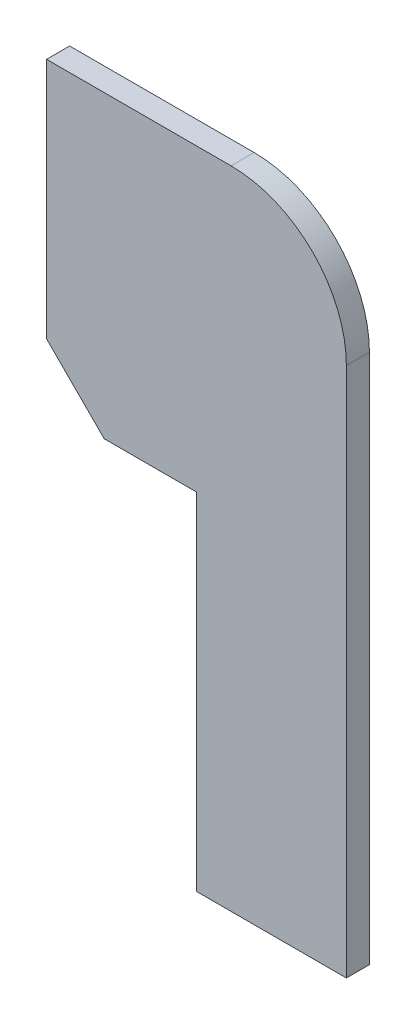
SolidWorks part; units mm, degrees
material "普通碳钢"
ref_plane "Front Plane" through (0, 0, 0) normal (0, 0, 1) x (1, 0, 0)
ref_plane "Top Plane" through (0, 0, 0) normal (0, 1, 0) x (1, 0, 0)
ref_plane "Right Plane" through (0, 0, 0) normal (1, 0, 0) x (0, 0, -1)
sketch "Sketch1" plane through (0, 0, 0) normal (0, 0, 1) x (1, 0, 0)
  line L0 (0, 175) -> (0, 280)
  line L1 (0, 280) -> (80, 280)
  line L2 (130, 230) -> (130, 0)
  line L3 (130, 0) -> (65, 0)
  line L4 (65, 0) -> (65, 150)
  line L5 (65, 150) -> (25, 150)
  line L6 (25, 150) -> (0, 175)
  arc A0 (80, 280) -> (130, 230) centre (80, 230) cw
  point P0 (0, 150)
  dimension "D5" = 50
  dimension "D1" = 280
  dimension "D2" = 150
  dimension "D3" = 65
  dimension "D4" = 130
extrude "Boss-Extrude1" add sketch "Sketch1" along normal mid plane 10
